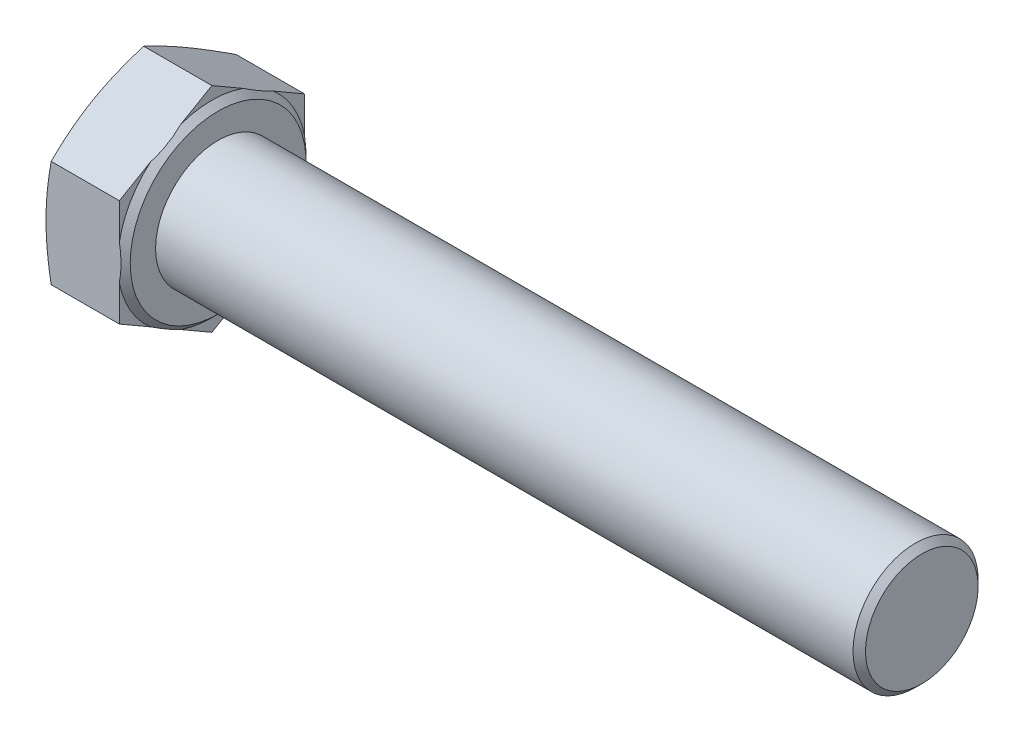
SolidWorks part; units mm, degrees
ref_plane "Front" through (0, 0, 0) normal (0, 0, 1) x (1, 0, 0)
ref_plane "Top" through (0, 0, 0) normal (0, 1, 0) x (1, 0, 0)
ref_plane "Right" through (0, 0, 0) normal (1, 0, 0) x (0, 0, -1)
sketch "Sketch2" plane through (0, 0, 0) normal (1, 0, 0) x (0, 0, -1)
  line L1 (11.835, -6.8329) -> (11.835, 6.8329)
  line L2 (11.835, 6.8329) -> (0, 13.6659)
  line L3 (0, 13.6659) -> (-11.835, 6.8329)
  line L4 (-11.835, 6.8329) -> (-11.835, -6.8329)
  line L5 (-11.835, -6.8329) -> (0, -13.6659)
  line L6 (0, -13.6659) -> (11.835, -6.8329)
  circle A0 centre (0, 0) radius 11.835 construction
extrude "BaseHead" add sketch "Sketch2" along normal blind 10.18
sketch "Sketch3" plane through (0, 0, 0) normal (0, 0, 1) x (1, 0, 0)
  line L0 (10.18, 13.6659) -> (10.18, 11.245)
  line L2 (10.18, 11.245) -> (9.38, 12.045)
  line L3 (9.38, 12.045) -> (9.38, 13.6659)
  line L5 (9.38, 13.6659) -> (10.18, 13.6659)
  line L6 (-0.9571, 0) -> (7.6478, 0) construction
  line L7 (10.18, 13.6659) -> (0, 13.6659) construction
  dimension "D1" = 45
  dimension "c" = 0.8
  dimension "Dw" = 22.49
revolve "BearingFace" cut sketch "Sketch3" angle 360 about L6
sketch "Sketch4" plane through (0, 0, 0) normal (0, 0, 1) x (1, 0, 0)
  line L0 (-0.4935, 0) -> (3.5626, 0) construction
  line L2 (0, 13.6659) -> (0.6664, 13.6659)
  line L4 (0.6664, 13.6659) -> (0, 11.835)
  line L6 (0, 11.835) -> (0, 13.6659)
  line L7 (9.38, 13.6659) -> (0, 13.6659) construction
revolve "Head chamfer" cut sketch "Sketch4" angle 360 about L0
sketch "Sketch5" plane through (10.18, 0, 0) normal (1, 0, 0) x (0, 0, -1)
  circle A0 centre (0, 0) radius 8
extrude "BaseBody" add sketch "Sketch5" along normal blind 90
cosmetic thread "Cosmetic thread1" [suppressed] parameters "D2"=13.835
chamfer "Chamfer1" distance 0.8 angle 45 1 edges at (100.18, 0, -8)
fillet "HeadFillet" [suppressed] radius 0.6
sketch "Sketch6" plane through (0, 0, 0) normal (0, 0, 1) x (1, 0, 0)
  line L0 (10.18, 9.0825) -> (11.2625, 9.0825)
  line L1 (11.2625, 9.0825) -> (11.2625, 8)
  line L2 (11.2625, 8) -> (10.7213, 7.0625)
  line L3 (10.7213, 7.0625) -> (10.18, 8)
  line L4 (10.18, 8) -> (10.18, 9.0825)
  line L5 (99.38, 8) -> (10.18, 8) construction
  line L6 (10.18, -11.245) -> (10.18, 11.245) construction
revolve "Cut-Revolve10" [suppressed] cut sketch "Sketch6" angle 360 about axis through (-0.9571, 0, 0) along (1, 0, 0)
pattern_linear "LPattern10" [suppressed] count 69
equation "\"D2@Sketch4\" = \"s@Sketch2\""
equation "\"D1@Chamfer1\" = 0.05 * \"d@Sketch5\""
equation "\"D1@Sketch6\" =  ( \"d@Sketch5\" - \"D2@Cosmetic thread1\" )  / 2"
equation "\"pitch@LPattern10\" = \"D1@Sketch6\" * 1.2"
equation "\"D1@LPattern10\" = \"l@BaseBody\" / \"pitch@LPattern10\""
